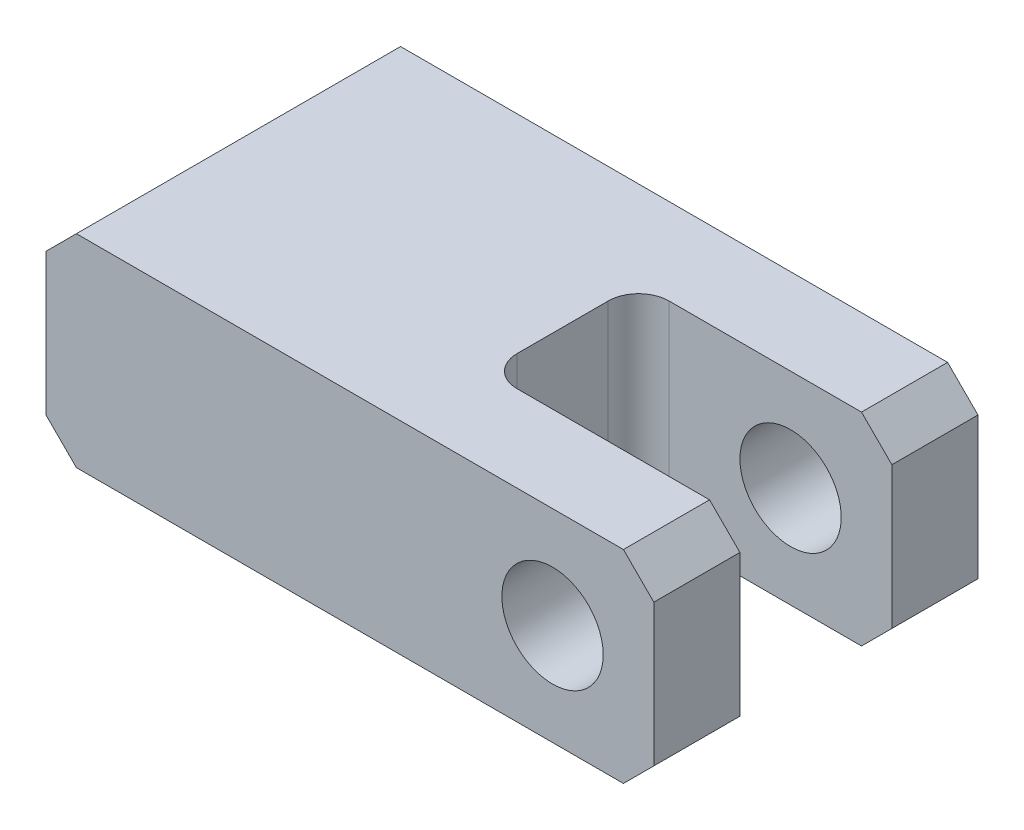
SolidWorks part; units mm, degrees
ref_plane "Front Plane" through (0, 0, 0) normal (0, 0, 1) x (1, 0, 0)
ref_plane "Top Plane" through (0, 0, 0) normal (0, 1, 0) x (1, 0, 0)
ref_plane "Right Plane" through (0, 0, 0) normal (1, 0, 0) x (0, 0, -1)
other "Configuration Table"
sketch "Sketch1" plane through (0, 0, 0) normal (0, 1, 0) x (1, 0, 0)
  line L1 (-30, 16) -> (30, 16)
  line L2 (-30, 16) -> (-30, -16)
  line L3 (-30, -16) -> (30, -16)
  line L4 (30, 16) -> (30, -16)
  line L5 (-30, 16) -> (30, -16) construction
  line L6 (-30, -16) -> (30, 16) construction
  point P0 (0, 0)
  dimension "D1" = 60
  dimension "D2" = 32
extrude "Boss-Extrude1" add sketch "Sketch1" along normal blind 20 contours L1 L4 L3 L2
sketch "Sketch2" plane through (0, 0, 16) normal (0, 0, 1) x (1, 0, 0)
  line L0 (-30, 0) -> (30, 0) construction
  line L1 (30, 20) -> (30, 0) construction
  circle A0 centre (20, 10) radius 5
  dimension "D3" = 10
  dimension "D1" = 10
  dimension "D2" = 10
extrude "Cut-Extrude1" cut sketch "Sketch2" against normal blind 42
chamfer "Chamfer1" distance 3 angle 45 4 edges at (-30, 0, 0) (-30, 20, 0) (30, 0, 0) (30, 20, 0)
hole_wizard "M6 Tapped Hole1" positions "Sketch4" profile "Sketch5" tap size "M6" standard "GB"
sketch "Sketch4" plane through (-30, 0, 0) normal (-1, 0, 0) x (0, 0, 1)
  line L0 (-16, 20) -> (16, 20) construction
  point P0 (-10, 10)
  point P2 (10, 10)
  dimension "D1" = 20
  dimension "D2" = 10
  dimension "D3" = 10
sketch "Sketch5" plane through (-30, 10, -10) normal (0, 1, 0) x (0, 0, 1)
  line L0 (0, 0) -> (0, 16.5022)
  line L1 (0, 16.5022) -> (2.5, 15)
  line L2 (2.5, 15) -> (2.5, 0)
  line L5 (2.5, 0) -> (0, 0)
  line L10 (0, 16.5022) -> (-2.5, 15) construction
  line L11 (0, -6.35) -> (0, 107.95) construction
  dimension "螺纹孔钻头直径" = 5
  dimension "螺纹孔钻头深度" = 15
  dimension "导头角度" = 118
cosmetic thread "Cosmetic Thread1" parameters "D1"=12, "D2"=6
cosmetic thread "Cosmetic Thread2" parameters "D1"=12, "D2"=6
sketch "Sketch6" plane through (30, 0, 0) normal (1, 0, 0) x (0, 0, -1)
  line L1 (-7.5, 25) -> (7.5, 25)
  line L2 (-7.5, 25) -> (-7.5, -5)
  line L3 (-7.5, -5) -> (7.5, -5)
  line L4 (7.5, 25) -> (7.5, -5)
  line L5 (-7.5, 25) -> (7.5, -5) construction
  line L6 (-7.5, -5) -> (7.5, 25) construction
  point P0 (0, 10)
  dimension "D1" = 15
  dimension "D2" = 30
  dimension "D3" = 10
extrude "Cut-Extrude2" cut sketch "Sketch6" against normal blind 25
fillet "Fillet1" radius 3 2 edges at (5, 10, 7.5) (5, 10, -7.5)
